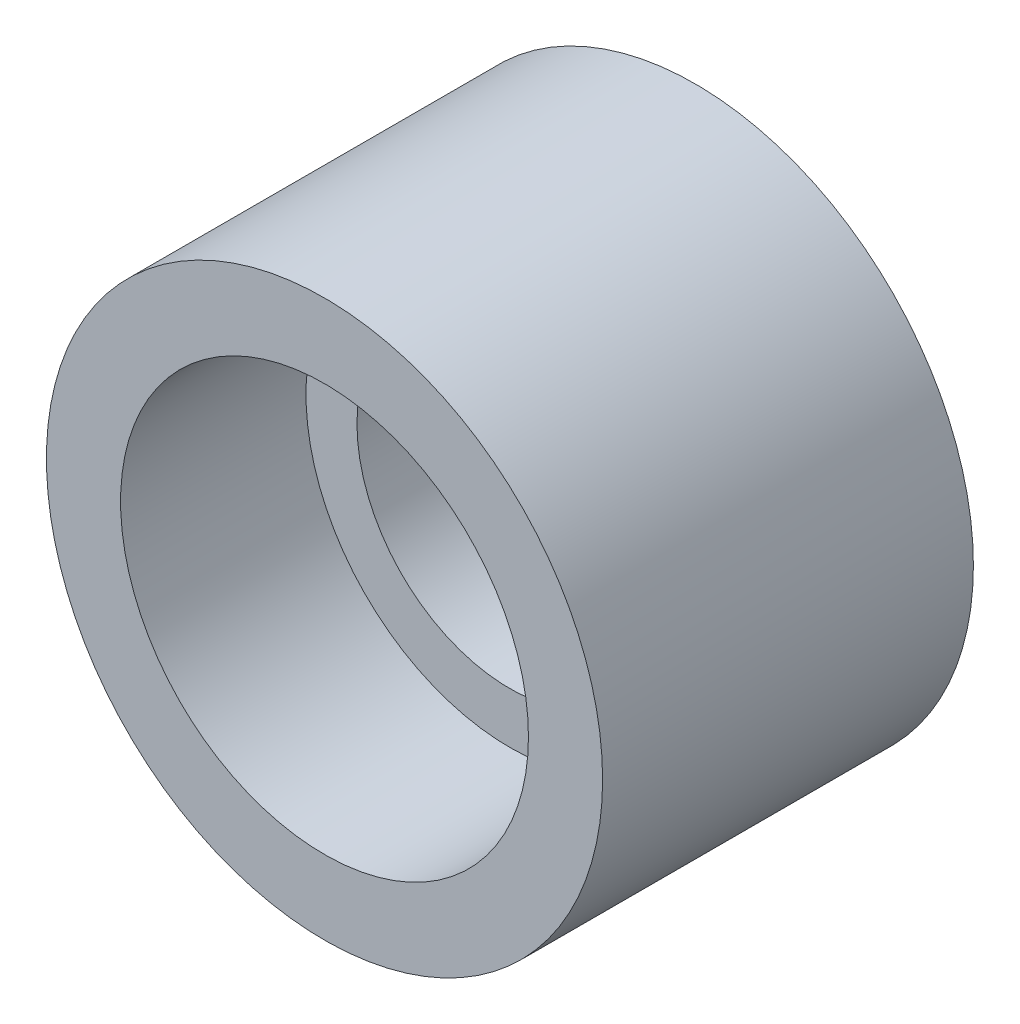
SolidWorks part; units mm, degrees
material "Q235B"
ref_plane "Front Plane" through (0, 0, 0) normal (0, 0, 1) x (1, 0, 0)
ref_plane "Top Plane" through (0, 0, 0) normal (0, 1, 0) x (1, 0, 0)
ref_plane "Right Plane" through (0, 0, 0) normal (1, 0, 0) x (0, 0, -1)
sketch "Sketch1" plane through (0, 0, 0) normal (0, 0, 1) x (1, 0, 0)
  circle A0 centre (0, 0) radius 15
  dimension "D1" = 30
extrude "Boss-Extrude1" add sketch "Sketch1" along normal blind 20
sketch "Sketch2" plane through (0, 0, 20) normal (0, 0, 1) x (1, 0, 0)
  circle A0 centre (0, 0) radius 11
  dimension "D1" = 22
extrude "Cut-Extrude1" cut sketch "Sketch2" against normal blind 10
hole_wizard "M18x1.5 Tapped Hole1" positions "Sketch3" profile "Sketch4" tap size "M18x1.5" standard "GB"
sketch "Sketch3" plane through (0, 0, 0) normal (0, 0, -1) x (-1, 0, 0)
  point P0 (0, 0)
sketch "Sketch4" plane through (0, 0, 0) normal (1, 0, 0) x (0, 1, 0)
  line L0 (0, 0) -> (0, 45.4571)
  line L1 (0, 45.4571) -> (8.25, 40.5)
  line L2 (8.25, 40.5) -> (8.25, 0)
  line L5 (8.25, 0) -> (0, 0)
  line L10 (0, 45.4571) -> (-8.25, 40.5) construction
  line L11 (0, -6.35) -> (0, 107.95) construction
  dimension "螺纹孔钻头直径" = 16.5
  dimension "螺纹孔钻头深度" = 40.5
  dimension "导头角度" = 118
cosmetic thread "Cosmetic thread 1"
